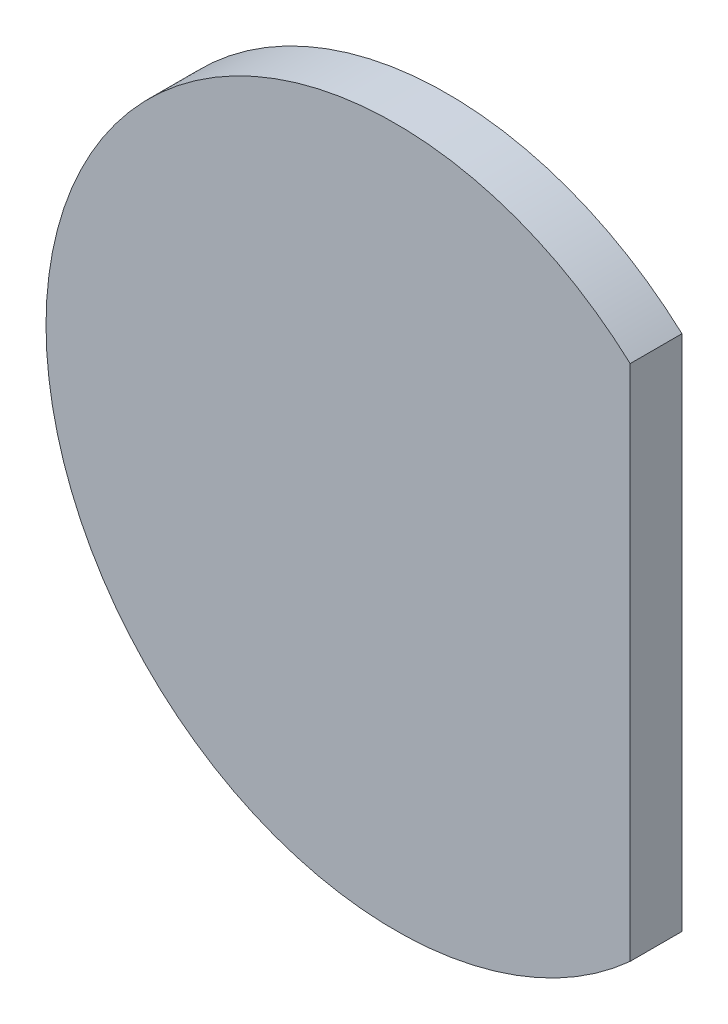
from build123d import *

# Parameters (mm, degrees)
BOSS_EXTRUDE1_DEPTH = 20


with BuildPart() as part:
    # Sketch1 → Boss-Extrude1 (new body)
    with BuildSketch(Plane.XY):
        with BuildLine():
            Line((90.69, 100.001619487), (90.69, -100.001619487))
            ThreePointArc((90.69, -100.001619487), (-135, 0), (90.69, 100.001619487))
        make_face()
    extrude(amount=BOSS_EXTRUDE1_DEPTH)


solid = part.part
